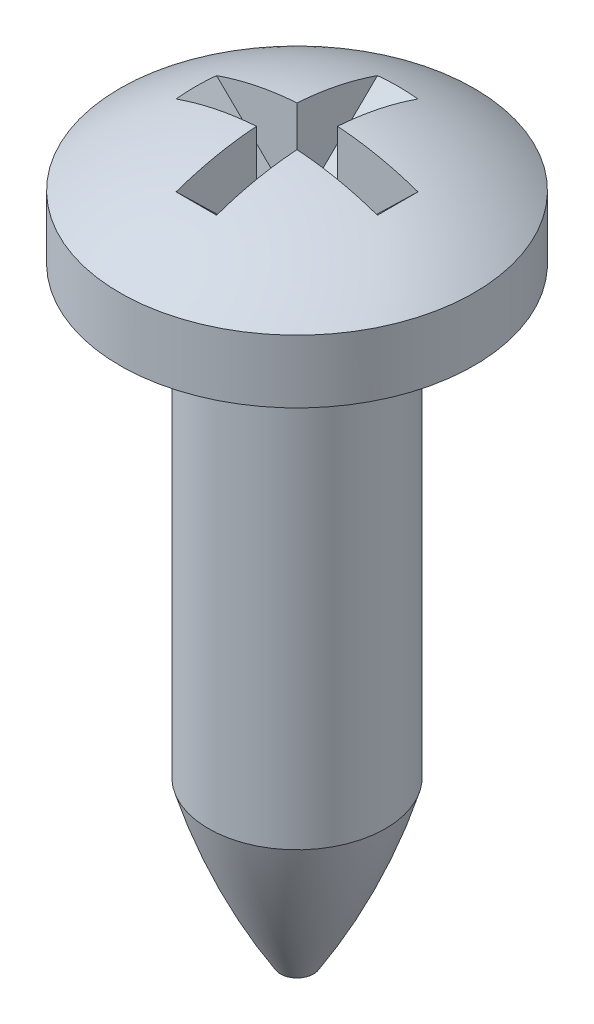
SolidWorks part; units mm, degrees
ref_plane "Front Plane" through (0, 0, 0) normal (0, 0, 1) x (1, 0, 0)
ref_plane "Top Plane" through (0, 0, 0) normal (0, 1, 0) x (1, 0, 0)
ref_plane "Right Plane" through (0, 0, 0) normal (1, 0, 0) x (0, 0, -1)
other "Configuration Table"
sketch "Sketch1" plane through (0, 0, 0) normal (0, 0, 1) x (1, 0, 0)
  line L0 (0, 9.919) -> (0, 6.2313) construction
  line L1 (0, 3.8597) -> (3.5, 3.8597)
  line L2 (3.5, 3.8597) -> (3.5, 5.1047)
  line L6 (0, 6.2313) -> (0, 3.8597)
  line L7 (0, 3.8597) -> (0, -10.749) construction
  arc A0 (3.5, 5.1047) -> (0, 6.2313) centre (0, 0.2313) ccw
  dimension "D2" = 12
  dimension "D1" = 7
revolve "Revolve2" add sketch "Sketch1" angle 360 about L0
sketch "Sketch2" plane through (0, 3.8597, 0) normal (0, -1, 0) x (1, 0, 0)
  circle A0 centre (0, 0) radius 1.75
  dimension "D1" = 3.5
extrude "Boss-Extrude1" add sketch "Sketch2" along normal blind 8.8
sketch "Sketch3" plane through (0, 0, 0) normal (0, 0, 1) x (1, 0, 0)
  line L0 (0, 0) -> (0, -8.1403) construction
  line L2 (-1.75, -4.9403) -> (1.75, -4.9403) construction
  line L3 (-0.3269, -8.1403) -> (0, -8.1403)
  line L4 (0, -4.9403) -> (-1.75, -4.9403)
  line L5 (0, -4.9403) -> (0, -8.1403)
  arc A0 (-1.75, -4.9403) -> (-0.3269, -8.1403) centre (10.5472, -1.3879) ccw
  dimension "D3" = 25.6
  dimension "D2" = 3.2
revolve "Revolve3" add sketch "Sketch3" angle 360 about L0
sketch "Sketch8" plane through (0, 0, 0) normal (0, 0, 1) x (1, 0, 0)
  line L1 (-2, 5.8882) -> (-0.4, 4.3313)
  line L2 (-0.4, 4.3313) -> (0.4, 4.3313)
  line L3 (0.4, 4.3313) -> (2, 5.8882)
  arc A1 (2, 5.8882) -> (-2, 5.8882) centre (0, 0.2313) ccw
  dimension "D1" = 0.8
  dimension "D2" = 4
extrude "Cut-Extrude1" cut sketch "Sketch8" against normal mid plane 0.8
pattern_circular "CirPattern1" count 4 over 360 about axis through (0, 0, 0) along (0, 1, 0) of "Cut-Extrude1"
